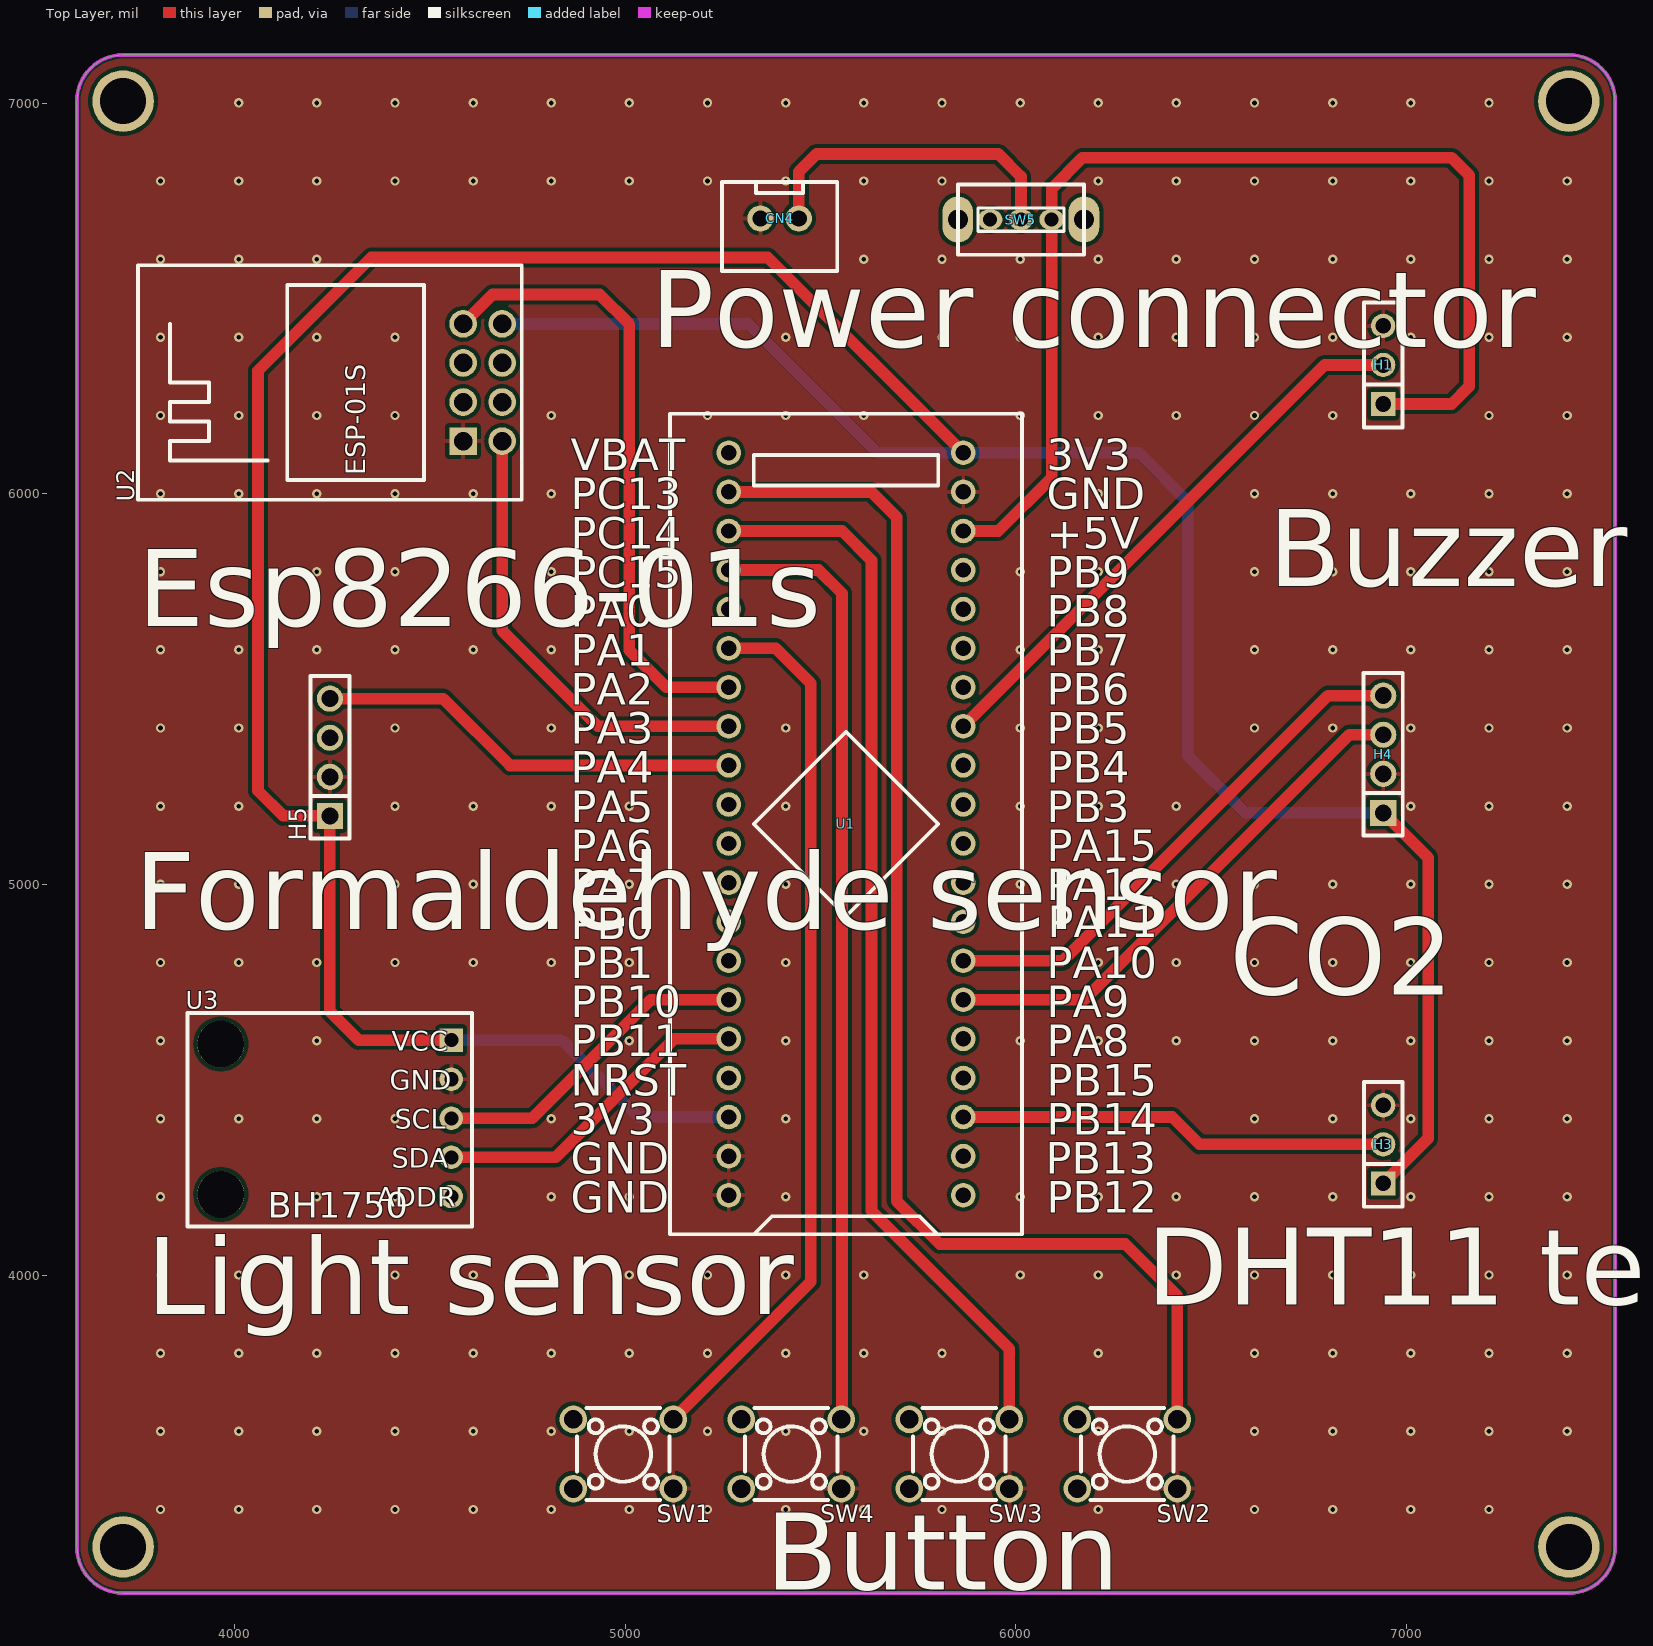
[diagram p0: Top Layer view]
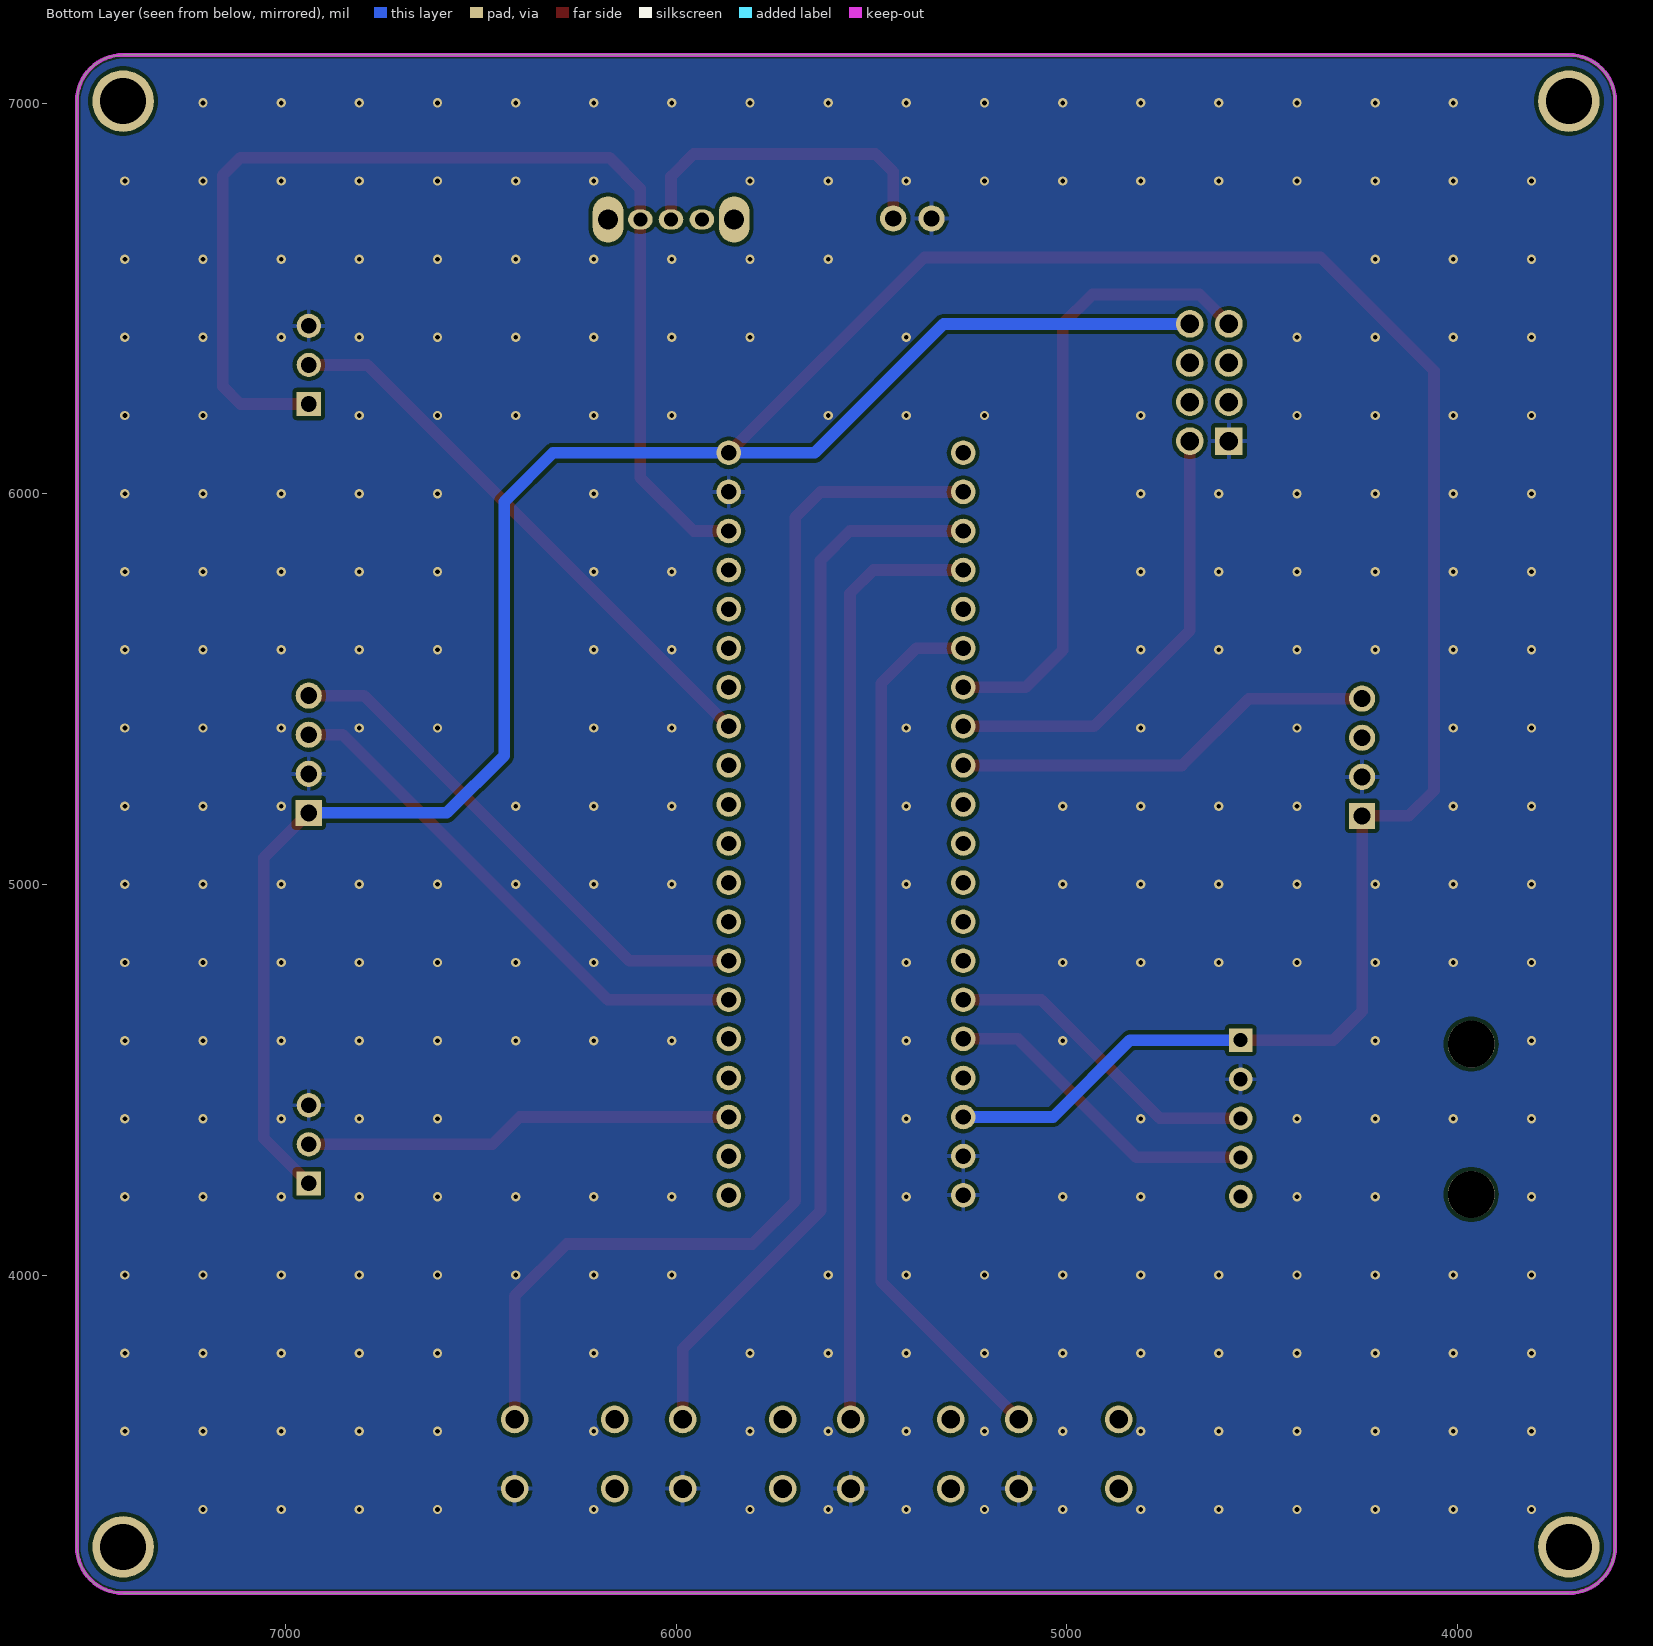
[diagram p1: Bottom Layer view, seen from below]
# Altium PCB MISC51847.pcbdoc
Units mil, origin at the board's own origin, x right, y up, seen from the top; angles counter-clockwise.
Board outline 3937.01 x 3937.01 mil, 2 copper layers (Top Layer, Bottom Layer), stack 62.206 mil thick; 13 components, 38 nets, 96 pads, 276 vias.

## Layer stack, top to bottom
Top Solder Mask Layer: solder mask 0.394, Dk 3.3
Top Layer: signal copper 1.379
Dielectric1: surface 59.449, FR4, Dk 4.5
Bottom Layer: signal copper 1.378
Bottom Solder Mask Layer: solder mask 0.394, Dk 3.3

## Board outline
3714.61,7123.5 ccw(c3714.61,7005.39) 3596.5,7005.39 3596.5,3304.61 ccw(c3714.61,3304.61) 3714.61,3186.5 7415.39,3186.5 ccw(c7415.39,3304.61) 7533.5,3304.61 7533.5,7005.39 ccw(c7415.39,7005.39) 7415.39,7123.5 3714.61,7123.5

## Design rules (kind name [scope] priority, off if disabled: settings)
BoardOutlineClearance copperThickness2oz_1 [All] p2 off: genericclearance=7.99 ignorepadtopadclearanceinfootprint=FALSE except(0: Arc-SplitContinuation Track-SplitContinuation SMDPad-SplitContinuation THPad-SplitContinuation Via-SplitContinuation Fill-SplitContinuation Region-SplitContinuation Poly-SplitContinuation Text-SplitContinuation Hole-SplitContinuation; 5.98: Arc-CutoutEdge Track-CutoutEdge SMDPad-CutoutEdge THPad-CutoutEdge Via-CutoutEdge Text-CutoutEdge; 6.9: Hole-OutlineEdge Hole-CutoutEdge; 10: Poly-OutlineEdge Poly-CutoutEdge; 11.81: Arc-OutlineEdge Track-OutlineEdge SMDPad-OutlineEdge THPad-OutlineEdge Via-OutlineEdge Fill-OutlineEdge Region-OutlineEdge Text-OutlineEdge Fill-CutoutEdge Region-CutoutEdge)
BoardOutlineClearance Plane_innerPlane_1 [All] p4 off: genericclearance=4.02 ignorepadtopadclearanceinfootprint=FALSE except(0: Arc-SplitContinuation Track-SplitContinuation SMDPad-SplitContinuation THPad-SplitContinuation Via-SplitContinuation Fill-SplitContinuation Region-SplitContinuation Poly-SplitContinuation Text-SplitContinuation Hole-SplitContinuation; 5.98: Arc-CutoutEdge Track-CutoutEdge SMDPad-CutoutEdge THPad-CutoutEdge Via-CutoutEdge Text-CutoutEdge; 6.9: Hole-OutlineEdge Hole-CutoutEdge; 10: Poly-OutlineEdge Poly-CutoutEdge; 11.81: Arc-OutlineEdge Track-OutlineEdge SMDPad-OutlineEdge THPad-OutlineEdge Via-OutlineEdge Fill-OutlineEdge Region-OutlineEdge Text-OutlineEdge Fill-CutoutEdge Region-CutoutEdge)
BoardOutlineClearance Copper_copperRegion_1 [All] p6 off: genericclearance=4.02 ignorepadtopadclearanceinfootprint=FALSE except(0: Arc-SplitContinuation Track-SplitContinuation SMDPad-SplitContinuation THPad-SplitContinuation Via-SplitContinuation Fill-SplitContinuation Region-SplitContinuation Poly-SplitContinuation Text-SplitContinuation Hole-SplitContinuation; 5.98: Arc-CutoutEdge Track-CutoutEdge SMDPad-CutoutEdge THPad-CutoutEdge Via-CutoutEdge Text-CutoutEdge; 6.9: Hole-OutlineEdge Hole-CutoutEdge; 10: Poly-OutlineEdge Poly-CutoutEdge; 11.81: Arc-OutlineEdge Track-OutlineEdge SMDPad-OutlineEdge THPad-OutlineEdge Via-OutlineEdge Fill-OutlineEdge Region-OutlineEdge Text-OutlineEdge Fill-CutoutEdge Region-CutoutEdge)
BoardOutlineClearance Copper_copperRegion_copperThickness1oz_1 [All] p8 off: genericclearance=4.02 ignorepadtopadclearanceinfootprint=FALSE except(0: Arc-SplitContinuation Track-SplitContinuation SMDPad-SplitContinuation THPad-SplitContinuation Via-SplitContinuation Fill-SplitContinuation Region-SplitContinuation Poly-SplitContinuation Text-SplitContinuation Hole-SplitContinuation; 5.98: Arc-CutoutEdge Track-CutoutEdge SMDPad-CutoutEdge THPad-CutoutEdge Via-CutoutEdge Text-CutoutEdge; 6.9: Hole-OutlineEdge Hole-CutoutEdge; 10: Poly-OutlineEdge Poly-CutoutEdge; 11.81: Arc-OutlineEdge Track-OutlineEdge SMDPad-OutlineEdge THPad-OutlineEdge Via-OutlineEdge Fill-OutlineEdge Region-OutlineEdge Text-OutlineEdge Fill-CutoutEdge Region-CutoutEdge)
BoardOutlineClearance Copper_copperRegion_Copper_copperRegion_1 [All] p10 off: genericclearance=4.02 ignorepadtopadclearanceinfootprint=FALSE except(0: Arc-SplitContinuation Track-SplitContinuation SMDPad-SplitContinuation THPad-SplitContinuation Via-SplitContinuation Fill-SplitContinuation Region-SplitContinuation Poly-SplitContinuation Text-SplitContinuation Hole-SplitContinuation; 5.98: Arc-CutoutEdge Track-CutoutEdge SMDPad-CutoutEdge THPad-CutoutEdge Via-CutoutEdge Text-CutoutEdge; 6.9: Hole-OutlineEdge Hole-CutoutEdge; 10: Poly-OutlineEdge Poly-CutoutEdge; 11.81: Arc-OutlineEdge Track-OutlineEdge SMDPad-OutlineEdge THPad-OutlineEdge Via-OutlineEdge Fill-OutlineEdge Region-OutlineEdge Text-OutlineEdge Fill-CutoutEdge Region-CutoutEdge)
BoardOutlineClearance copperThickness1oz_1 [All] p12: genericclearance=4.02 ignorepadtopadclearanceinfootprint=FALSE except(0: Arc-SplitContinuation Track-SplitContinuation SMDPad-SplitContinuation THPad-SplitContinuation Via-SplitContinuation Fill-SplitContinuation Region-SplitContinuation Poly-SplitContinuation Text-SplitContinuation Hole-SplitContinuation; 5.98: Arc-CutoutEdge Track-CutoutEdge SMDPad-CutoutEdge THPad-CutoutEdge Via-CutoutEdge Text-CutoutEdge; 6.9: Hole-OutlineEdge Hole-CutoutEdge; 10: Poly-OutlineEdge Poly-CutoutEdge; 11.81: Arc-OutlineEdge Track-OutlineEdge SMDPad-OutlineEdge THPad-OutlineEdge Via-OutlineEdge Fill-OutlineEdge Region-OutlineEdge Text-OutlineEdge Fill-CutoutEdge Region-CutoutEdge)
Clearance copperThickness2oz [All] p1 off: gap=7.99 ignorepadtopadclearanceinfootprint=FALSE except(5.98: SMDPad-Track SMDPad-SMDPad THPad-Track SMDPad-THPad THPad-THPad Track-Via SMDPad-Via THPad-Via Via-Via Fill-SMDPad Region-SMDPad Fill-THPad Region-THPad Fill-Via Region-Via Fill-Fill Fill-Region Region-Region Arc-Track Arc-SMDPad Arc-THPad Arc-Via Fill-Arc Region-Arc Arc-Arc Text-Track SMDPad-Text Text-THPad Text-Via Fill-Text Region-Text Arc-Text Text-Text; 6.9: Hole-Track Hole-SMDPad Hole-THPad Hole-Via Fill-Hole Region-Hole Hole-Arc Hole-Text; 10: Poly-Track Poly-SMDPad Poly-THPad Poly-Via Poly-Fill Poly-Region Poly-Poly Poly-Arc Poly-Text Poly-Hole; 11.81: Fill-Track Region-Track)
Clearance Plane_innerPlane [All] p3 off: gap=4.02 ignorepadtopadclearanceinfootprint=FALSE except(5.98: SMDPad-Track SMDPad-SMDPad THPad-Track SMDPad-THPad THPad-THPad Track-Via SMDPad-Via THPad-Via Via-Via Fill-SMDPad Region-SMDPad Fill-THPad Region-THPad Fill-Via Region-Via Fill-Fill Fill-Region Region-Region Arc-Track Arc-SMDPad Arc-THPad Arc-Via Fill-Arc Region-Arc Arc-Arc Text-Track SMDPad-Text Text-THPad Text-Via Fill-Text Region-Text Arc-Text Text-Text; 6.9: Hole-Track Hole-SMDPad Hole-THPad Hole-Via Fill-Hole Region-Hole Hole-Arc Hole-Text; 10: Poly-Track Poly-SMDPad Poly-THPad Poly-Via Poly-Fill Poly-Region Poly-Poly Poly-Arc Poly-Text Poly-Hole; 11.81: Fill-Track Region-Track)
Clearance Copper_copperRegion [All] p5 off: gap=4.02 ignorepadtopadclearanceinfootprint=FALSE except(5.98: SMDPad-Track SMDPad-SMDPad THPad-Track SMDPad-THPad THPad-THPad Track-Via SMDPad-Via THPad-Via Via-Via Fill-SMDPad Region-SMDPad Fill-THPad Region-THPad Fill-Via Region-Via Fill-Fill Fill-Region Region-Region Arc-Track Arc-SMDPad Arc-THPad Arc-Via Fill-Arc Region-Arc Arc-Arc Text-Track SMDPad-Text Text-THPad Text-Via Fill-Text Region-Text Arc-Text Text-Text; 6.9: Hole-Track Hole-SMDPad Hole-THPad Hole-Via Fill-Hole Region-Hole Hole-Arc Hole-Text; 10: Poly-Track Poly-SMDPad Poly-THPad Poly-Via Poly-Fill Poly-Region Poly-Poly Poly-Arc Poly-Text Poly-Hole; 11.81: Fill-Track Region-Track)
Clearance Copper_copperRegion_copperThickness1oz [All] p7 off: gap=4.02 ignorepadtopadclearanceinfootprint=FALSE except(5.98: SMDPad-Track SMDPad-SMDPad THPad-Track SMDPad-THPad THPad-THPad Track-Via SMDPad-Via THPad-Via Via-Via Fill-SMDPad Region-SMDPad Fill-THPad Region-THPad Fill-Via Region-Via Fill-Fill Fill-Region Region-Region Arc-Track Arc-SMDPad Arc-THPad Arc-Via Fill-Arc Region-Arc Arc-Arc Text-Track SMDPad-Text Text-THPad Text-Via Fill-Text Region-Text Arc-Text Text-Text; 6.9: Hole-Track Hole-SMDPad Hole-THPad Hole-Via Fill-Hole Region-Hole Hole-Arc Hole-Text; 10: Poly-Track Poly-SMDPad Poly-THPad Poly-Via Poly-Fill Poly-Region Poly-Poly Poly-Arc Poly-Text Poly-Hole; 11.81: Fill-Track Region-Track)
Clearance Copper_copperRegion_Copper_copperRegion [All] p9 off: gap=4.02 ignorepadtopadclearanceinfootprint=FALSE except(5.98: SMDPad-Track SMDPad-SMDPad THPad-Track SMDPad-THPad THPad-THPad Track-Via SMDPad-Via THPad-Via Via-Via Fill-SMDPad Region-SMDPad Fill-THPad Region-THPad Fill-Via Region-Via Fill-Fill Fill-Region Region-Region Arc-Track Arc-SMDPad Arc-THPad Arc-Via Fill-Arc Region-Arc Arc-Arc Text-Track SMDPad-Text Text-THPad Text-Via Fill-Text Region-Text Arc-Text Text-Text; 6.9: Hole-Track Hole-SMDPad Hole-THPad Hole-Via Fill-Hole Region-Hole Hole-Arc Hole-Text; 10: Poly-Track Poly-SMDPad Poly-THPad Poly-Via Poly-Fill Poly-Region Poly-Poly Poly-Arc Poly-Text Poly-Hole; 11.81: Fill-Track Region-Track)
Clearance copperThickness1oz [All] p11: gap=4.02 ignorepadtopadclearanceinfootprint=FALSE except(5.98: SMDPad-Track SMDPad-SMDPad THPad-Track SMDPad-THPad THPad-THPad Track-Via SMDPad-Via THPad-Via Via-Via Fill-SMDPad Region-SMDPad Fill-THPad Region-THPad Fill-Via Region-Via Fill-Fill Fill-Region Region-Region Arc-Track Arc-SMDPad Arc-THPad Arc-Via Fill-Arc Region-Arc Arc-Arc Text-Track SMDPad-Text Text-THPad Text-Via Fill-Text Region-Text Arc-Text Text-Text; 6.9: Hole-Track Hole-SMDPad Hole-THPad Hole-Via Fill-Hole Region-Hole Hole-Arc Hole-Text; 10: Poly-Track Poly-SMDPad Poly-THPad Poly-Via Poly-Fill Poly-Region Poly-Poly Poly-Arc Poly-Text Poly-Hole; 11.81: Fill-Track Region-Track)
DiffPairsRouting differentialPair [All] p1: maxlimit=6 minlimit=6 mostfreqgap=6 toplayer_minwidth=5 toplayer_prefwidth=10 toplayer_maxwidth=100 toplayer_mingap=6 toplayer_prefgap=6 toplayer_maxgap=6 bottomlayer_minwidth=5 bottomlayer_prefwidth=10 bottomlayer_maxwidth=100 bottomlayer_mingap=6 bottomlayer_prefgap=6 bottomlayer_maxgap=6 maxuncoupledlength=10
HoleToHoleClearance otherClearance [All] p1: gap=11.81 allowstackedmicrovias=TRUE
Length netLength [All] p1: minlimit=0 maxlimit=0
PasteMaskExpansion pasteMaskExpansion [All] p1: expansion=0
PlaneConnect innerPlane [All] p1: planeconnectstyle=Relief reliefexpansion=20 reliefentries=4 reliefconductorwidth=10 reliefairgap=10
PolygonConnect copperRegion_copperThickness1oz [All] p1 off: connectstyle=Relief reliefconductorwidth=10 reliefentries=4 polygonreliefangle="90 Angle" airgapwidth=10 via.connectstyle=Relief via.reliefconductorwidth=10 via.reliefentries=4 via.polygonreliefangle="90 Angle" via.airgapwidth=10
PolygonConnect copperRegion_Copper_copperRegion [All] p2 off: connectstyle=Relief reliefconductorwidth=10 reliefentries=4 polygonreliefangle="90 Angle" airgapwidth=10 via.connectstyle=Relief via.reliefconductorwidth=10 via.reliefentries=4 via.polygonreliefangle="90 Angle" via.airgapwidth=10
PolygonConnect copperRegion [All] p3: connectstyle=Relief reliefconductorwidth=10 reliefentries=4 polygonreliefangle="90 Angle" airgapwidth=10 via.connectstyle=Relief via.reliefconductorwidth=10 via.reliefentries=4 via.polygonreliefangle="90 Angle" via.airgapwidth=10
RoutingVias viaSize [All] p1: holewidth=12.01 width=24.02 viastyle="Through Hole" minholewidth=11.81 minwidth=19.68 maxholewidth=248.03 maxwidth=393.7
SolderMaskExpansion solderMaskExpansion [IsVia] p1: expansion=-1000 istentingtop=TRUE
SolderMaskExpansion solderMaskExpansion [All] p2: expansion=2 istentingtop=FALSE
Width copperThickness2oz_2 [All] p1 off: maxlimit=100 minlimit=8 preferedwidth=10
Width copperThickness1oz_2 [All] p2: maxlimit=100 minlimit=5 preferedwidth=10

## Components (designator, comment, footprint, x,y, rotation, side; value= is the part's Value field where it differs from the comment)
CN4 "XH2.54*2P_Through-hole" CONN-TH_2P-P2.50-XH2.54-2P 5395,6705 r0 top
H1 "" HDR-TH_3P-P2.54-V-F 6940,6330 r90 top
H3 "" HDR-TH_3P-P2.54-V-F 6940,4335.16 r90 top
H4 "" HDR-TH_4P-P2.54-V-F 6940,5333.47 r90 top
H5 "" HDR-TH_4P-P2.54-V-F 4244,5325.8 r90 top
SW1 "" SW-TH_4P-L6.0-W6.0-P4.50-LS6.5 4995,3542.47 r180 top
SW2 "" SW-TH_4P-L6.0-W6.0-P4.50-LS6.5 6285,3542.47 r180 top
SW3 "" SW-TH_4P-L6.0-W6.0-P4.50-LS6.5 5855,3542.47 r180 top
SW4 "" SW-TH_4P-L6.0-W6.0-P4.50-LS6.5 5425,3542.47 r180 top
SW5 "" 拨动开关 6017.9,6702.05 r180 top
U1 "STM32F103C8T6-Card" CONN-TH_L53.3-W22.9_STM32F103C8T6-CARD 5565,5155 r90 top
U2 "ESP-01S" WIFIM-TH_ESP-01S 4635,6285 r90 top
U3 "" BH1750光照传感器 4294.83,4391.77 r0 top

## Footprints (in the part's own frame and the unit in brackets; to place one, negate y for a bottom-side part, rotate by r counter-clockwise, add the part's x,y. Pads: shape width x height; smd on the part's side, far side on the other; paste and mask are expansions set on the pad)
BH1750光照传感器 [mil]
  rect 60x60 hole 36: 1(260,210)
  round 60 hole 36: 2(260,110) 3(260,10) 4(260,-90) 5(260,-190)
  round 120 hole 120 unplated: ""(-330,-185) ""(-330,200)
  silkscreen extent -415,-267 313,280
CONN-TH_2P-P2.50-XH2.54-2P [mm]
  round 1.7 hole 1.05 paste+0 mask+0.05: 1(1.25,0) 2(-1.25,0)
  silkscreen extent -3.75,-3.42 3.75,2.37
CONN-TH_L53.3-W22.9_STM32F103C8T6-CARD [mm]
  round 1.6 hole 1: 1(-24.13,-7.62) 2(-21.59,-7.62) 3(-19.05,-7.62) 4(-16.51,-7.62) 5(-13.97,-7.62) 6(-11.43,-7.62) 7(-8.89,-7.62) 8(-6.35,-7.62) 9(-3.81,-7.62) 10(-1.27,-7.62) 11(1.27,-7.62) 12(3.81,-7.62) 13(6.35,-7.62) 14(8.89,-7.62) 15(11.43,-7.62) 16(13.97,-7.62) 17(16.51,-7.62) 18(19.05,-7.62) 19(21.59,-7.62) 20(24.13,-7.62) 21(24.13,7.62) 22(21.59,7.62) 23(19.05,7.62) 24(16.51,7.62) 25(13.97,7.62) 26(11.43,7.62) 27(8.89,7.62) 28(6.35,7.62) 29(3.81,7.62) 30(1.27,7.62) 31(-1.27,7.62) 32(-3.81,7.62) 33(-6.35,7.62) 34(-8.89,7.62) 35(-11.43,7.62) 36(-13.97,7.62) 37(-16.51,7.62) 38(-19.05,7.62) 39(-21.59,7.62) 40(-24.13,7.62)
  silkscreen extent -26.67,-11.43 26.67,11.43
HDR-TH_3P-P2.54-V-F [mil]
  rect 62x62 hole 40.16: 1(-100,0)
  round 62 hole 40.16: 2(0,0) 3(100,0)
  silkscreen extent -160,-49 160,49
HDR-TH_4P-P2.54-V-F [mm]
  rect 1.7x1.7 hole 1.1: 1(-3.81,0)
  round 1.7 hole 1.1: 2(-1.27,0) 3(1.27,0) 4(3.81,0)
  silkscreen extent -5.29,-1.27 5.29,1.27
SW-TH_4P-L6.0-W6.0-P4.50-LS6.5 [mm]
  round 1.8 hole 1.2: 1(-3.25,2.25) 2(3.25,2.25) 3(-3.25,-2.25) 4(3.25,-2.25)
  silkscreen extent -3,-3 3,3
WIFIM-TH_ESP-01S [mm]
  rect 1.8x1.8 hole 1.2: 1(-3.81,1.27)
  round 1.8 hole 1.2: 2(-1.27,1.27) 3(1.27,1.27) 4(3.81,1.27) 5(3.81,-1.27) 6(1.27,-1.27) 7(-1.27,-1.27) 8(-3.81,-1.27)
  silkscreen extent -7.62,-2.54 7.62,22.4
拨动开关 [mil]
  oval 63x51.2 hole 35.4 paste+0 mask+2: 1(-73.4,0) 2(5,0) 3(84,0)
  oval 78.7x118.1 hole 51.2 paste+0 mask+2: 4(166.7,0) 5(-156.1,0)
  silkscreen extent -156,-90 167,90

## Free pads (board coordinates)
  round 157.48 hole 118.11: 1(3714.61,7005.39) 1(3714.61,3304.61) 1(7415.39,7005.39) 1(7415.39,3304.61)

## Via types
v1: diameter 24.02, hole 12, Top Layer to Bottom Layer, 276 vias

## Nets (pads, with @x,y where several pads share a name; then routed paths per layer and width w, separated by ;. In a path a pad name is that pad's centre, name@x,y a point inside that pad or via, vN(x,y) a via of type N, cw(c..) or ccw(c..) an arc to the next point about the centre after c; other vN are vias at no path point)
$1N17118: CN4.1 SW5.2 | length 840.9
  Top Layer w30: CN4.1 5444.22,6824.22 5490,6870 5955,6870 6012.9,6812.1 SW5.2
+5V: H1.1 SW5.1 U1.18 | length 2921.3
  Top Layer w30: U1.18 5955,5905 6091.3,6041.3 SW5.1 6091.3,6781.3 6170,6860 7115,6860 7160,6815 7160,6275 7115,6230 H1.1
GND: CN4.2 H1.3 H3.3 H4.2 H5.2 SW1.1 SW2.1 SW3.1 SW4.1 U1.19 U1.39 U1.40 U2.1 U3.2
  other v1: 3810.6,3400.6 4010.6,3400.6 4210.6,3400.6 4410.6,3400.6 4610.6,3400.6 4810.6,3400.6 5010.6,3400.6 5210.6,3400.6 5410.6,3400.6 5610.6,3400.6 5810.6,3400.6 6210.6,3400.6 6610.6,3400.6 6810.6,3400.6 7010.6,3400.6 7210.6,3400.6 3810.6,3600.6 4010.6,3600.6 4210.6,3600.6 4410.6,3600.6 4610.6,3600.6 4810.6,3600.6 5010.6,3600.6 5210.6,3600.6 5410.6,3600.6 5610.6,3600.6 5810.6,3600.6 6210.6,3600.6 6610.6,3600.6 6810.6,3600.6 7010.6,3600.6 7210.6,3600.6 7410.6,3600.6 3810.6,3800.6 4010.6,3800.6 4210.6,3800.6 4410.6,3800.6 4610.6,3800.6 4810.6,3800.6 5010.6,3800.6 5210.6,3800.6 5410.6,3800.6 5610.6,3800.6 5810.6,3800.6 6210.6,3800.6 6610.6,3800.6 6810.6,3800.6 7010.6,3800.6 7210.6,3800.6 7410.6,3800.6 3810.6,4000.6 4010.6,4000.6 4210.6,4000.6 4410.6,4000.6 4610.6,4000.6 4810.6,4000.6 5010.6,4000.6 5210.6,4000.6 5410.6,4000.6 5610.6,4000.6 6010.6,4000.6 6210.6,4000.6 6410.6,4000.6 6610.6,4000.6 6810.6,4000.6 7010.6,4000.6 7210.6,4000.6 7410.6,4000.6 3810.6,4200.6 4210.6,4200.6 4410.6,4200.6 4810.6,4200.6 5010.6,4200.6 5410.6,4200.6 6010.6,4200.6 6210.6,4200.6 6410.6,4200.6 6610.6,4200.6 6810.6,4200.6 7010.6,4200.6 7210.6,4200.6 7410.6,4200.6 3810.6,4400.6 4010.6,4400.6 4210.6,4400.6 4410.6,4400.6 4810.6,4400.6 5410.6,4400.6 6610.6,4400.6 6810.6,4400.6 7010.6,4400.6 7210.6,4400.6 7410.6,4400.6 3810.6,4600.6 4210.6,4600.6 5010.6,4600.6 5410.6,4600.6 6010.6,4600.6 6210.6,4600.6 6410.6,4600.6 6610.6,4600.6 6810.6,4600.6 7010.6,4600.6 7210.6,4600.6 7410.6,4600.6 3810.6,4800.6 4010.6,4800.6 4210.6,4800.6 4410.6,4800.6 4610.6,4800.6 4810.6,4800.6 5010.6,4800.6 5410.6,4800.6 6210.6,4800.6 6410.6,4800.6 6610.6,4800.6 6810.6,4800.6 7010.6,4800.6 7210.6,4800.6 7410.6,4800.6 3810.6,5000.6 4010.6,5000.6 4210.6,5000.6 4410.6,5000.6 4610.6,5000.6 4810.6,5000.6 5010.6,5000.6 5410.6,5000.6 6010.6,5000.6 6210.6,5000.6 6410.6,5000.6 6610.6,5000.6 6810.6,5000.6 7010.6,5000.6 7210.6,5000.6 7410.6,5000.6 3810.6,5200.6 4010.6,5200.6 4410.6,5200.6 4610.6,5200.6 4810.6,5200.6 5010.6,5200.6 5410.6,5200.6 6010.6,5200.6 6210.6,5200.6 6410.6,5200.6 7010.6,5200.6 7210.6,5200.6 7410.6,5200.6 3810.6,5400.6 4010.6,5400.6 4410.6,5400.6 4810.6,5400.6 5410.6,5400.6 6010.6,5400.6 6210.6,5400.6 6610.6,5400.6 6810.6,5400.6 7010.6,5400.6 7210.6,5400.6 7410.6,5400.6 3810.6,5600.6 4010.6,5600.6 4210.6,5600.6 4410.6,5600.6 4610.6,5600.6 4810.6,5600.6 6010.6,5600.6 6210.6,5600.6 6610.6,5600.6 6810.6,5600.6 7010.6,5600.6 7210.6,5600.6 7410.6,5600.6 3810.6,5800.6 4010.6,5800.6 4210.6,5800.6 4410.6,5800.6 4610.6,5800.6 4810.6,5800.6 6010.6,5800.6 6210.6,5800.6 6610.6,5800.6 6810.6,5800.6 7010.6,5800.6 7210.6,5800.6 7410.6,5800.6 3810.6,6000.6 4010.6,6000.6 4210.6,6000.6 4410.6,6000.6 4610.6,6000.6 4810.6,6000.6 6210.6,6000.6 6610.6,6000.6 6810.6,6000.6 7010.6,6000.6 7210.6,6000.6 7410.6,6000.6 3810.6,6200.6 4010.6,6200.6 4210.6,6200.6 4410.6,6200.6 4810.6,6200.6 5210.6,6200.6 5410.6,6200.6 5610.6,6200.6 6010.6,6200.6 6210.6,6200.6 6410.6,6200.6 6610.6,6200.6 6810.6,6200.6 7210.6,6200.6 7410.6,6200.6 3810.6,6400.6 4010.6,6400.6 4210.6,6400.6 4410.6,6400.6 5410.6,6400.6 5810.6,6400.6 6010.6,6400.6 6210.6,6400.6 6410.6,6400.6 6610.6,6400.6 6810.6,6400.6 7010.6,6400.6 7210.6,6400.6 7410.6,6400.6 3810.6,6600.6 4010.6,6600.6 4210.6,6600.6 5610.6,6600.6 5810.6,6600.6 6010.6,6600.6 6210.6,6600.6 6410.6,6600.6 6610.6,6600.6 6810.6,6600.6 7010.6,6600.6 7210.6,6600.6 7410.6,6600.6 3810.6,6800.6 4010.6,6800.6 4210.6,6800.6 4410.6,6800.6 4610.6,6800.6 4810.6,6800.6 5010.6,6800.6 5210.6,6800.6 5410.6,6800.6 5610.6,6800.6 5810.6,6800.6 6210.6,6800.6 6410.6,6800.6 6610.6,6800.6 6810.6,6800.6 7010.6,6800.6 7210.6,6800.6 7410.6,6800.6 4010.6,7000.6 4210.6,7000.6 4410.6,7000.6 4610.6,7000.6 4810.6,7000.6 5010.6,7000.6 5210.6,7000.6 5410.6,7000.6 5610.6,7000.6 5810.6,7000.6 6010.6,7000.6 6210.6,7000.6 6410.6,7000.6 6610.6,7000.6 6810.6,7000.6 7010.6,7000.6 7210.6,7000.6
NRST: U1.37
PA0: U1.25
PA1: SW1.3 U1.26 | length 2277.1
  Top Layer w30: SW1.3 5475,3983.1 5475,5515 5385,5605 U1.26
PA2: U1.27 U2.4 | length 1616.5
  Top Layer w30: U2.4 4660,6510 4935,6510 5010,6435 5010,5600 5105,5505 U1.27
PA3: U1.28 U2.8 | length 1166.5
  Top Layer w30: U2.8 4685,5650 4930,5405 U1.28
PA4: H5.4 U1.29 | length 1091.7
  Top Layer w30: H5.4 4534.2,5475.8 4705,5305 U1.29
PA5: U1.30
PA6: U1.31
PA7: U1.32
PA8: U1.5
PA9: H4.3 U1.6 | length 1356
  Top Layer w30: U1.6 6175,4705 6853.47,5383.47 H4.3
PA10: H4.4 U1.7 | length 1356
  Top Layer w30: U1.7 6120,4805 6798.47,5483.47 H4.4
PA11: U1.8
PA12: U1.9
PA15: U1.10
PB0: U1.33
PB1: U1.34
PB3: U1.11
PB4: U1.12
PB5: H1.2 U1.13 | length 1458.1
  Top Layer w30: U1.13 6790,6330 H1.2
PB6: U1.14
PB7: U1.15
PB8: U1.16
PB9: U1.17
PB10: U1.35 U3.3 | length 835.8
  Top Layer w30: U3.3 4761.77,4401.77 5065,4705 U1.35
PB11: U1.36 U3.4 | length 835.8
  Top Layer w30: U3.4 4821.77,4301.77 5125,4605 U1.36
PB12: U1.1
PB13: U1.2
PB14: H3.2 U1.3 | length 1103.9
  Top Layer w30: U1.3 6400,4405 6469.84,4335.16 H3.2
PB15: U1.4
PC13: SW2.3 U1.22 | length 3341.5
  Top Layer w30: U1.22 5630,6005 5695,5940 5695,4190 5805,4080 6280,4080 6412.95,3947.05 SW2.3
PC14: SW3.3 U1.23 | length 2741.2
  Top Layer w30: U1.23 5555,5905 5630,5830 5630,4165 5982.95,3812.05 SW3.3
PC15: SW4.3 U1.24 | length 2429.7
  Top Layer w30: U1.24 5495,5805 5555,5745 5555,3633.1 SW4.3
VBAT: U1.21
VCC: H3.1 H4.1 H5.1 U1.20 U1.38 U2.5 U3.1 | length 9248.6
  Top Layer w30: U3.1 4318.23,4601.77 4244,4676 H5.1 4124.2,5175.8 4060,5240 4060,6315 4350,6605 5365,6605 U1.20 ; H3.1 7055,4350.16 7055,5068.47 H4.1
  Bottom Layer w30: U3.1 4838.23,4601.77 5035,4405 U1.38 ; U2.5 5315,6435 5645,6105 U1.20 6315,6105 6440,5980 6440,5330 6586.53,5183.47 H4.1
pads on no net: H5.3 SW1.2 SW1.4 SW2.2 SW2.4 SW3.2 SW3.4 SW4.2 SW4.4 SW5.3 SW5.4 SW5.5 U2.2 U2.3 U2.6 U2.7 U3. U3.5

## Polygon pours and split planes (outlines as drawn)
GND on Bottom Layer (solid, remove dead copper, pour order 2): 3525,7245 3525,3080 7700,3080 7700,7245
GND on Top Layer (solid, remove dead copper, pour order 2): 3000,7415 3000,3000 7930,3000 7930,7415

## Keep-outs
Board Outline Layer:
  the board outline again, w10

## Silkscreen, mask and mechanical layers (free items; w line width, h text height)
Top Silkscreen Layer:
  text "Power connector" at 5065,6375 h196.85
  text "VBAT" at 4860.95,6060 h80
  text "3V3" at 6079.16,6060 h80
  text "PC13" at 4860.95,5960 h80
  text "GND" at 6079.16,5960 h80
  text "PC14" at 4860.95,5860 h80
  text "+5V" at 6079.16,5860 h80
  text "Buzzer" at 6646.81,5764.09 h196.85
  text "PC15" at 4860.95,5760 h80
  text "PB9" at 6079.16,5760 h80
  text "Esp8266-01s" at 3752.02,5661.06 h196.85
  text "PA0" at 4860.95,5660 h80
  text "PB8" at 6079.16,5660 h80
  text "PA1" at 4860.95,5560 h80
  text "PB7" at 6079.16,5560 h80
  text "PA2" at 4860.95,5460 h80
  text "PB6" at 6079.16,5460 h80
  text "PA3" at 4860.95,5360 h80
  text "PB5" at 6079.16,5360 h80
  text "PA4" at 4860.95,5260 h80
  text "PB4" at 6079.16,5260 h80
  text "PA5" at 4860.95,5160 h80
  text "PB3" at 6079.16,5160 h80
  text "PA6" at 4860.95,5060 h80
  text "PA15" at 6079.16,5060 h80
  text "PA7" at 4860.95,4960 h80
  text "PA12" at 6079.16,4960 h80
  text "Formaldehyde sensor" at 3745,4885 h196.85
  text "PA11" at 6080.95,4865 h80
  text "PB0" at 4860.95,4860 h80
  text "PB1" at 4860.95,4760 h80
  text "PA10" at 6079.16,4760 h80
  text "CO2" at 6546.75,4718.54 h196.85
  text "PB10" at 4860.95,4660 h80
  text "PA9" at 6079.16,4660 h80
  text "PB11" at 4860.95,4560 h80
  text "PA8" at 6079.16,4560 h80
  text "NRST" at 4860.95,4460 h80
  text "PB15" at 6079.16,4460 h80
  text "3V3" at 4860.95,4360 h80
  text "PB14" at 6079.16,4360 h80
  text "GND" at 4860.95,4260 h80
  text "PB13" at 6075.95,4260 h80
  text "GND" at 4860.95,4160 h80
  text "PB12" at 6079.16,4160 h80
  text "DHT11 temp/humidity" at 6335,3925 h196.85
  text "Light sensor" at 3775,3900 h196.85
  text "Button" at 5360,3195 h196.85